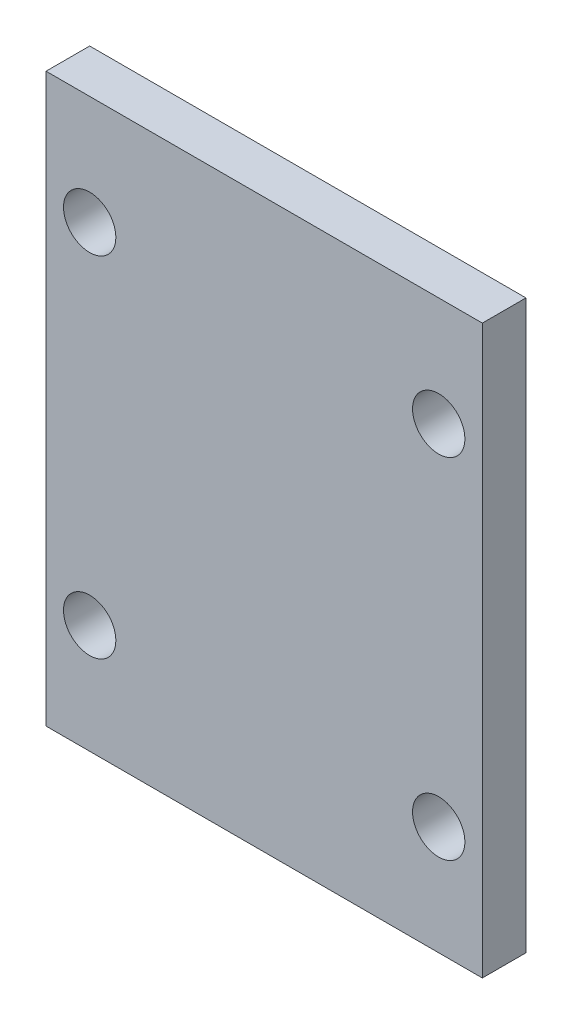
SolidWorks part; units mm, degrees
material "Q235B"
ref_plane "Front Plane" through (0, 0, 0) normal (0, 0, 1) x (1, 0, 0)
ref_plane "Top Plane" through (0, 0, 0) normal (0, 1, 0) x (1, 0, 0)
ref_plane "Right Plane" through (0, 0, 0) normal (1, 0, 0) x (0, 0, -1)
sketch "Sketch1" plane through (0, 0, 0) normal (0, 0, 1) x (1, 0, 0)
  line L1 (50, -65) -> (-50, -65)
  line L2 (50, -65) -> (50, 65)
  line L3 (50, 65) -> (-50, 65)
  line L4 (-50, -65) -> (-50, 65)
  line L5 (50, -65) -> (-50, 65) construction
  line L6 (50, 65) -> (-50, -65) construction
  point P0 (0, 0)
  dimension "D1" = 130
  dimension "D2" = 100
extrude "Boss-Extrude1" add sketch "Sketch1" along normal mid plane 10
hole_wizard "Ø12 Hole1" positions "Sketch2" profile "Sketch3" hole size "Ø12.0" standard "GB" end condition up to next
sketch "Sketch2" plane through (0, 0, 5) normal (0, 0, 1) x (1, 0, 0)
  line L0 (0, 65) -> (0, 0) construction
  line L1 (50, 65) -> (-50, 65) construction
  line L2 (0, 0) -> (-40, 0) construction
  point P0 (-40, 40)
  point P13 (40, 40)
  point P14 (40, -40)
  point P15 (-40, -40)
  dimension "D1" = 80
  dimension "D2" = 80
  dimension "D3" = 25
sketch "Sketch3" plane through (-40, 40, 5) normal (1, 0, 0) x (0, -1, 0)
  line L0 (0, 0) -> (0, 10)
  line L1 (0, 10) -> (6, 10)
  line L2 (6, 10) -> (6, 0)
  line L5 (6, 0) -> (0, 0)
  line L11 (0, -6.35) -> (0, 107.95) construction
  dimension "通孔孔直径" = 12
  dimension "通孔孔深度" = 10
chamfer "Chamfer1" [suppressed] distance 10 angle 45
